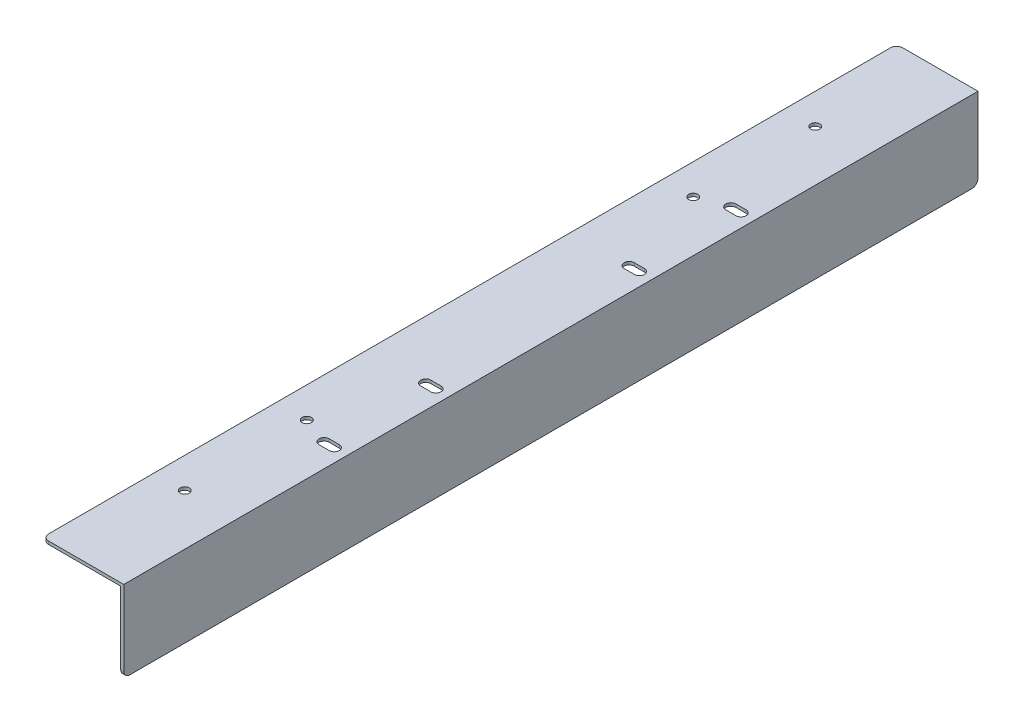
SolidWorks part; units mm, degrees
material "Q235"
ref_plane "前视基准面" through (0, 0, 0) normal (0, 0, 1) x (1, 0, 0)
ref_plane "上视基准面" through (0, 0, 0) normal (0, 1, 0) x (1, 0, 0)
ref_plane "右视基准面" through (0, 0, 0) normal (1, 0, 0) x (0, 0, -1)
sketch "草图1" plane through (0, 0, 0) normal (1, 0, 0) x (0, 0, -1)
  line L0 (-210, -20) -> (210, 20) construction
  line L1 (-210, 20) -> (210, 20)
  line L2 (-210, 20) -> (-210, -20)
  line L3 (-210, -20) -> (210, -20)
  line L4 (210, 20) -> (210, -20)
  line L5 (210, 20) -> (209.4475, 20) construction
  dimension "D1" = 420
  dimension "D2" = 40
extrude "凸台-拉伸1" add sketch "草图1" along normal blind 1.5
sketch "草图2" plane through (1.5, 0, 0) normal (1, 0, 0) x (0, 0, -1)
  line L1 (-210, 20) -> (210, 20)
  line L2 (-210, 20) -> (-210, 18.5)
  line L3 (-210, 18.5) -> (210, 18.5)
  line L4 (210, 20) -> (210, 18.5)
  line L5 (210, -20) -> (210, 20) construction
  dimension "D1" = 1.5
extrude "凸台-拉伸2" add sketch "草图2" against normal blind 40
fillet "圆角1" radius 3 4 edges at (-38.5, 19.25, -210) (0.75, -20, -210) (-38.5, 19.25, 210) (0.75, -20, 210)
sketch "草图3" plane through (0, 20, 0) normal (0, 1, 0) x (1, 0, 0)
  line L0 (1.5, 210) -> (1.5, -210) construction
  line L1 (1.5, -210) -> (-35.5, -210) construction
  line L2 (-38.5, 0) -> (1.5, 0) construction
  line L3 (-38.5, 207) -> (-38.5, -207) construction
  circle A0 centre (-23.5, -95) radius 2.25
  circle A1 centre (-23.5, 95) radius 2.25
  dimension "D1" = 4.5
  dimension "D2" = 25
  dimension "D3" = 115
extrude "切除-拉伸1" cut sketch "草图3" against normal blind 10
hole_wizard "M4 螺纹孔1" positions "3D草图1" profile "草图5" tap size "M4" standard "GB"
sketch3d "3D草图1"
  point P0 (0, -10, -150)
  point P2 (0, -10, 150)
  point P3 (0, -10, -160)
  point P5 (0, -10, 140)
  point P9 (0, -10, 130)
  point P11 (0, -10, -170)
  dimension "D1" = 60
  dimension "D2" = 10
  dimension "D3" = 60
  dimension "D4" = 10
  dimension "D5" = 10
  dimension "D6" = 10
  dimension "D7" = 10
  dimension "D8" = 10
sketch "草图5" plane through (0, -10, -150) normal (0, 1, 0) x (0, 0, 1)
  line L0 (0, 0) -> (0, 12.4914)
  line L1 (0, 12.4914) -> (1.65, 11.5)
  line L2 (1.65, 11.5) -> (1.65, 0)
  line L5 (1.65, 0) -> (0, 0)
  line L10 (0, 12.4914) -> (-1.65, 11.5) construction
  line L11 (0, -6.35) -> (0, 107.95) construction
  dimension "螺纹孔钻头直径" = 3.3
  dimension "螺纹孔钻头深度" = 11.5
  dimension "导头角度" = 118
cosmetic thread "孔螺蚊线1" [suppressed] parameters "D1"=2, "D2"=4
cosmetic thread "孔螺蚊线2" [suppressed] parameters "D1"=2, "D2"=4
cosmetic thread "孔螺蚊线3" [suppressed] parameters "D1"=2, "D2"=4
cosmetic thread "孔螺蚊线4" [suppressed] parameters "D1"=2, "D2"=4
cosmetic thread "孔螺蚊线5" [suppressed] parameters "D1"=2, "D2"=4
cosmetic thread "孔螺蚊线6" [suppressed] parameters "D1"=2, "D2"=4
sketch "草图6" plane through (0, 18.5, 0) normal (0, -1, 0) x (1, 0, 0)
  line L0 (1.5, 207) -> (1.5, -207) construction
  line L1 (-35.5, -210) -> (0, -210) construction
  line L2 (0, 0) -> (-38.0298, 0) construction
  circle A0 centre (-23.5, -155) radius 2.25
  circle A1 centre (-23.5, 155) radius 2.25
  dimension "D1" = 4.5
  dimension "D2" = 25
  dimension "D3" = 55
extrude "切除-拉伸2" cut sketch "草图6" against normal blind 10
sketch "草图7" plane through (0, 20, 0) normal (0, 1, 0) x (1, 0, 0)
  line L0 (-5.85, -100) -> (-9.15, -100) construction
  line L1 (-10, -100) -> (-5, -100) construction
  line L2 (-10, -97.5) -> (-5, -97.5)
  line L3 (-10, -102.5) -> (-5, -102.5)
  line L4 (-5, 50) -> (-10, 50) construction
  line L5 (-5, 47.5) -> (-10, 47.5)
  line L6 (-5, 52.5) -> (-10, 52.5)
  circle A0 centre (-7.5, -100) radius 1.65 construction
  arc A1 (-10, -97.5) -> (-10, -102.5) centre (-10, -100) ccw
  arc A2 (-5, -102.5) -> (-5, -97.5) centre (-5, -100) ccw
  arc A3 (-5, 47.5) -> (-5, 52.5) centre (-5, 50) ccw
  arc A4 (-10, 52.5) -> (-10, 47.5) centre (-10, 50) ccw
  point P7 (-7.5, -100)
  point P13 (-7.5, 50)
  dimension "D1" = 5
  dimension "D2" = 5
extrude "切除-拉伸3" cut sketch "草图7" against normal through all
ref_plane "基准面1" through (-13, 11, -208.5) normal (0, 0, -1) x (-1, 0, 0)
sketch "草图9" plane through (0, 20, 0) normal (0, 1, 0) x (1, 0, 0)
  line L0 (-5, -50) -> (-10, -50) construction
  line L1 (-5, -52.5) -> (-10, -52.5)
  line L2 (-5, -47.5) -> (-10, -47.5)
  line L3 (-5, 100) -> (-10, 100) construction
  line L4 (-5, 97.5) -> (-10, 97.5)
  line L5 (-5, 102.5) -> (-10, 102.5)
  arc A0 (-5, -52.5) -> (-5, -47.5) centre (-5, -50) ccw
  arc A1 (-10, -47.5) -> (-10, -52.5) centre (-10, -50) ccw
  arc A2 (-5, 97.5) -> (-5, 102.5) centre (-5, 100) ccw
  arc A3 (-10, 102.5) -> (-10, 97.5) centre (-10, 100) ccw
  point P4 (-7.5, -50)
  point P9 (-7.5, 100)
  dimension "D1" = 5
  dimension "D2" = 5
extrude "切除-拉伸4" cut sketch "草图9" against normal through all
